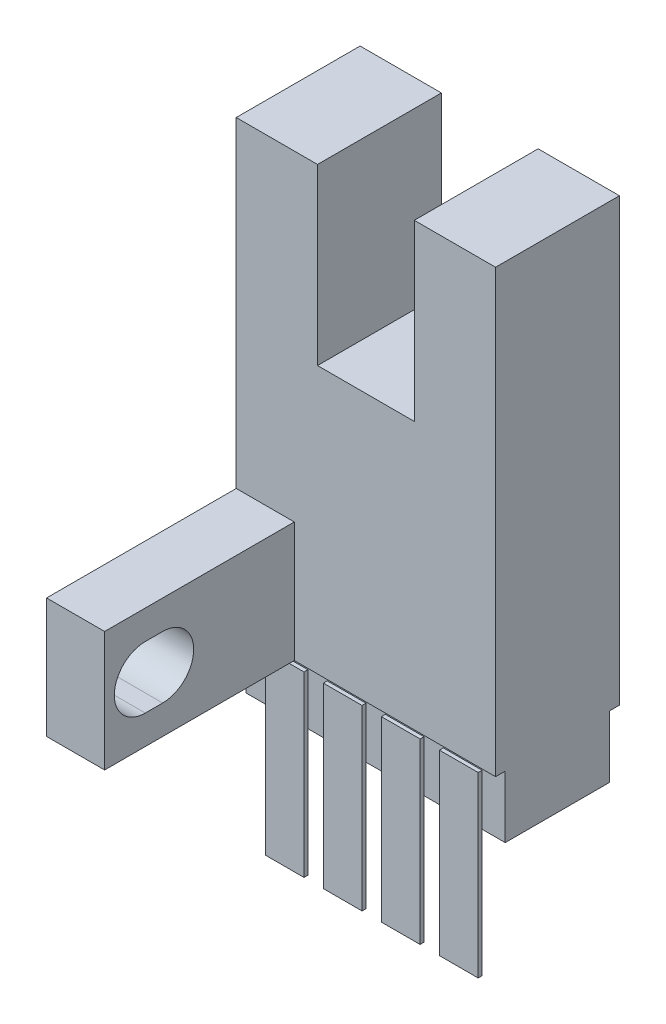
from build123d import *

# Parameters (mm, degrees)
SKETCH1_W           = 13.4
SKETCH1_H           = 26
BOSS_EXTRUDE1_DEPTH = 6.4
SKETCH2_W           = 5
SKETCH2_H           = 9
CUT_EXTRUDE1_DEPTH  = 30.941943825
SKETCH3_W           = 26
SKETCH3_H           = 6.2
BOSS_EXTRUDE2_DEPTH = 3
CUT_EXTRUDE2_DEPTH  = 34.436506995
SKETCH5_W           = 13.4
SKETCH5_H           = 3.2
CUT_EXTRUDE3_DEPTH  = 0.5
SKETCH6_W           = 13.4
SKETCH6_H           = 3.2
CUT_EXTRUDE4_DEPTH  = 0.5
SKETCH7_W           = 2
SKETCH7_H           = 9.197470194
BOSS_EXTRUDE3_DEPTH = 0.2
LPATTERN1_COUNT     = 4
LPATTERN1_PITCH     = 3


with BuildPart() as part:
    # Sketch1 → Boss-Extrude1 (new body)
    with BuildSketch(Plane.XY):
        with Locations((-6.7, 13)):
            Rectangle(SKETCH1_W, SKETCH1_H)
    extrude(amount=BOSS_EXTRUDE1_DEPTH)

    # Sketch2 → Cut-Extrude1 (cut, through all)
    with BuildSketch(Plane.XY.offset(6.4)):
        with Locations((-6.7, 21.5)):
            Rectangle(SKETCH2_W, SKETCH2_H)
    extrude(amount=-CUT_EXTRUDE1_DEPTH, mode=Mode.SUBTRACT)

    # Sketch3 → Boss-Extrude2 (add)
    with BuildSketch(Plane.ZY.offset(13.4)):
        with Locations((3.2, 6.3)):
            Rectangle(SKETCH3_W, SKETCH3_H)
    extrude(amount=-BOSS_EXTRUDE2_DEPTH)

    # Sketch4 → Cut-Extrude2 (cut, through all)
    with BuildSketch(Plane.ZY.offset(13.4)):
        with BuildLine():
            Line((-6.8, 7.9), (-5.9, 7.9))
            ThreePointArc((-5.9, 7.9), (-4.3, 6.3), (-5.9, 4.7))
            Line((-5.9, 4.7), (-6.8, 4.7))
            ThreePointArc((-6.8, 4.7), (-8.4, 6.3), (-6.8, 7.9))
        make_face()
        with BuildLine():
            Line((13.2, 7.9), (14.1, 7.9))
            ThreePointArc((14.1, 7.9), (15.7, 6.3), (14.1, 4.7))
            Line((14.1, 4.7), (13.2, 4.7))
            ThreePointArc((13.2, 4.7), (11.6, 6.3), (13.2, 7.9))
        make_face()
    extrude(amount=-CUT_EXTRUDE2_DEPTH, mode=Mode.SUBTRACT)

    # Sketch5 → Cut-Extrude3 (cut)
    with BuildSketch(Plane.XY.offset(6.4)):
        with Locations((-6.7, 1.6)):
            Rectangle(SKETCH5_W, SKETCH5_H)
    extrude(amount=-CUT_EXTRUDE3_DEPTH, mode=Mode.SUBTRACT)

    # Sketch6 → Cut-Extrude4 (cut)
    with BuildSketch(Plane(origin=(0, 0, 0), x_dir=(-1, 0, 0), z_dir=(0, 0, -1))):
        with Locations((6.7, 1.6)):
            Rectangle(SKETCH6_W, SKETCH6_H)
    extrude(amount=-CUT_EXTRUDE4_DEPTH, mode=Mode.SUBTRACT)

    # Sketch7 → Boss-Extrude3 (add)
    with BuildSketch(Plane.XY.offset(5.9)):
        with Locations((-2.2, -1.958933194)):
            Rectangle(SKETCH7_W, SKETCH7_H)
    boss_extrude3 = extrude(amount=BOSS_EXTRUDE3_DEPTH)

    # LPattern1: Boss-Extrude3 ×4
    with Locations(*[(-i * LPATTERN1_PITCH, 0, 0) for i in range(1, LPATTERN1_COUNT)]):
        add(boss_extrude3)


solid = part.part
